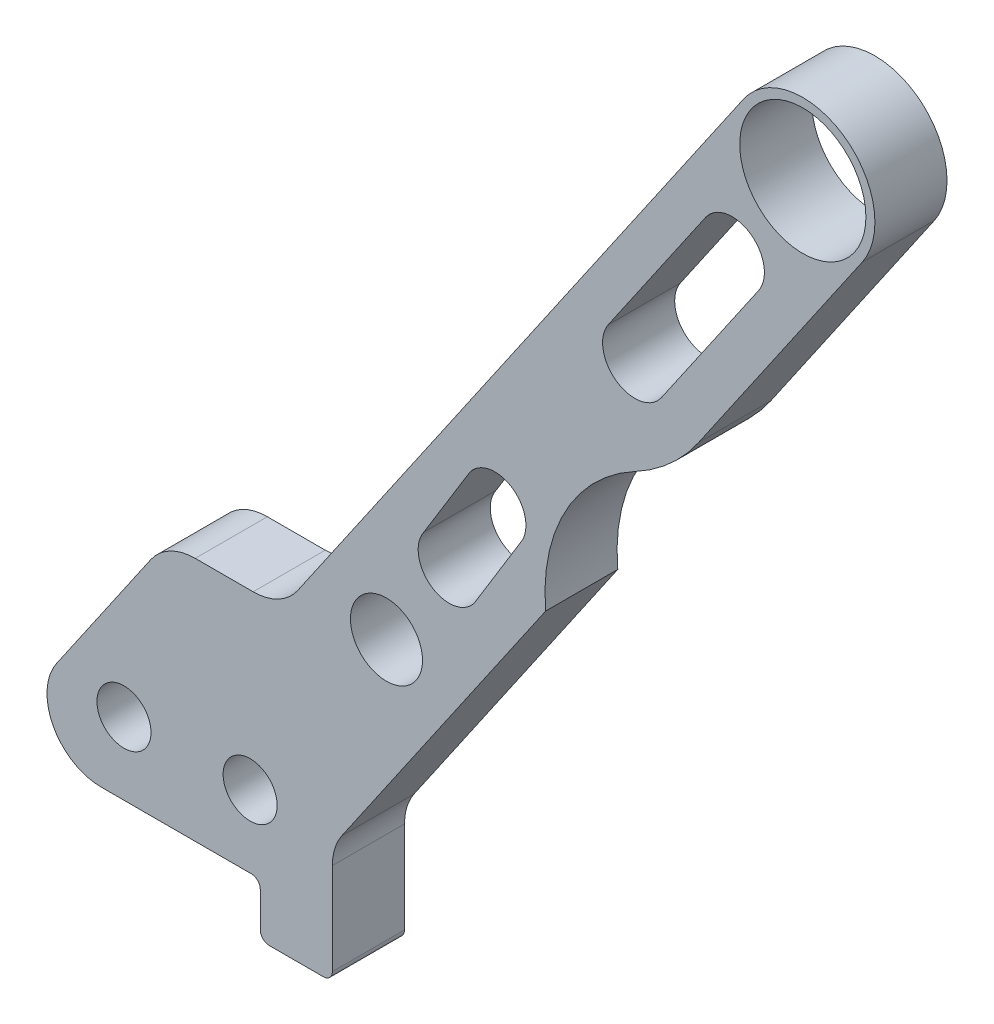
SolidWorks part; units mm, degrees
material "Q235B"
ref_plane "Front Plane" through (0, 0, 0) normal (0, 0, 1) x (1, 0, 0)
ref_plane "Top Plane" through (0, 0, 0) normal (0, 1, 0) x (1, 0, 0)
ref_plane "Right Plane" through (0, 0, 0) normal (1, 0, 0) x (0, 0, -1)
sketch "Sketch1" plane through (0, 0, 0) normal (0, 0, 1) x (1, 0, 0)
  line L0 (136298.4794, -173227.6312) -> (136051.2152, -173587.2882)
  line L1 (136364.4027, -173272.9536) -> (136273.6105, -173405.015)
  line L2 (136070.4411, -173760.7924) -> (136070.4411, -173709.8519)
  line L3 (135969.6368, -173613.2965) -> (135917.3868, -173689.2965)
  line L4 (135942.1081, -173736.2924) -> (136025.4411, -173736.2924)
  line L5 (136030.4411, -173760.7924) -> (136030.4411, -173741.2924)
  line L6 (136035.4411, -173765.7924) -> (136065.4411, -173765.7924)
  line L7 (135994.3581, -173600.2924) -> (136026.4939, -173600.2924)
  line L8 (136188.7812, -173528.403) -> (136075.7198, -173692.856)
  line L9 (136135.2426, -173534.2084) -> (136160.6387, -173492.7768) construction
  line L10 (136121.2266, -173524.2104) -> (136146.6939, -173482.7358)
  line L11 (136150.4739, -173542.2345) -> (136175.8481, -173500.7739)
  line L12 (136238.252, -173383.5932) -> (136292.231, -173305.0783) construction
  line L13 (136223.4946, -173373.4474) -> (136277.4736, -173294.9326)
  line L14 (136253.0094, -173393.7389) -> (136306.9884, -173315.224)
  circle A0 centre (136024.8161, -173696.2924) radius 15
  circle A1 centre (135954.8161, -173696.2924) radius 15
  arc A2 (136026.4939, -173600.2924) -> (136051.2152, -173587.2882) centre (136026.4939, -173570.2924) ccw
  arc A3 (135994.3581, -173600.2924) -> (135969.6368, -173613.2965) centre (135994.3581, -173630.2924) ccw
  arc A4 (135917.3868, -173689.2965) -> (135942.1081, -173736.2924) centre (135942.1081, -173706.2924) ccw
  arc A5 (136075.7198, -173692.856) -> (136070.4411, -173709.8519) centre (136100.4411, -173709.8519) ccw
  arc A6 (136065.4411, -173765.7924) -> (136070.4411, -173760.7924) centre (136065.4411, -173760.7924) ccw
  arc A7 (136030.4411, -173760.7924) -> (136035.4411, -173765.7924) centre (136035.4411, -173760.7924) ccw
  arc A8 (136030.4411, -173741.2924) -> (136025.4411, -173736.2924) centre (136025.4411, -173741.2924) ccw
  arc A9 (136364.4027, -173272.9536) -> (136298.4794, -173227.6312) centre (136331.4411, -173250.2924) ccw
  circle A10 centre (136100.4411, -173586.2924) radius 20
  circle A11 centre (136331.4411, -173250.2924) radius 35
  arc A12 (136121.2266, -173524.2104) -> (136150.4739, -173542.2345) centre (136135.2426, -173534.2084) ccw
  arc A13 (136175.8481, -173500.7739) -> (136146.6939, -173482.7358) centre (136160.6387, -173492.7768) ccw
  arc A14 (136223.4946, -173373.4474) -> (136253.0094, -173393.7389) centre (136238.252, -173383.5932) ccw
  arc A15 (136306.9884, -173315.224) -> (136277.4736, -173294.9326) centre (136292.231, -173305.0783) ccw
  arc A16 (136238.252, -173436.6044) -> (136273.6105, -173405.015) centre (136191.2063, -173348.3621) ccw
  arc A17 (136188.7812, -173528.403) -> (136238.252, -173436.6044) centre (136282.56, -173519.7116) cw
  point P2 (136156.7053, -173499.5524)
  point P39 (136265.2415, -173344.3357)
  dimension "D1" = 100
extrude "Boss-Extrude1" add sketch "Sketch1" along normal blind 40
